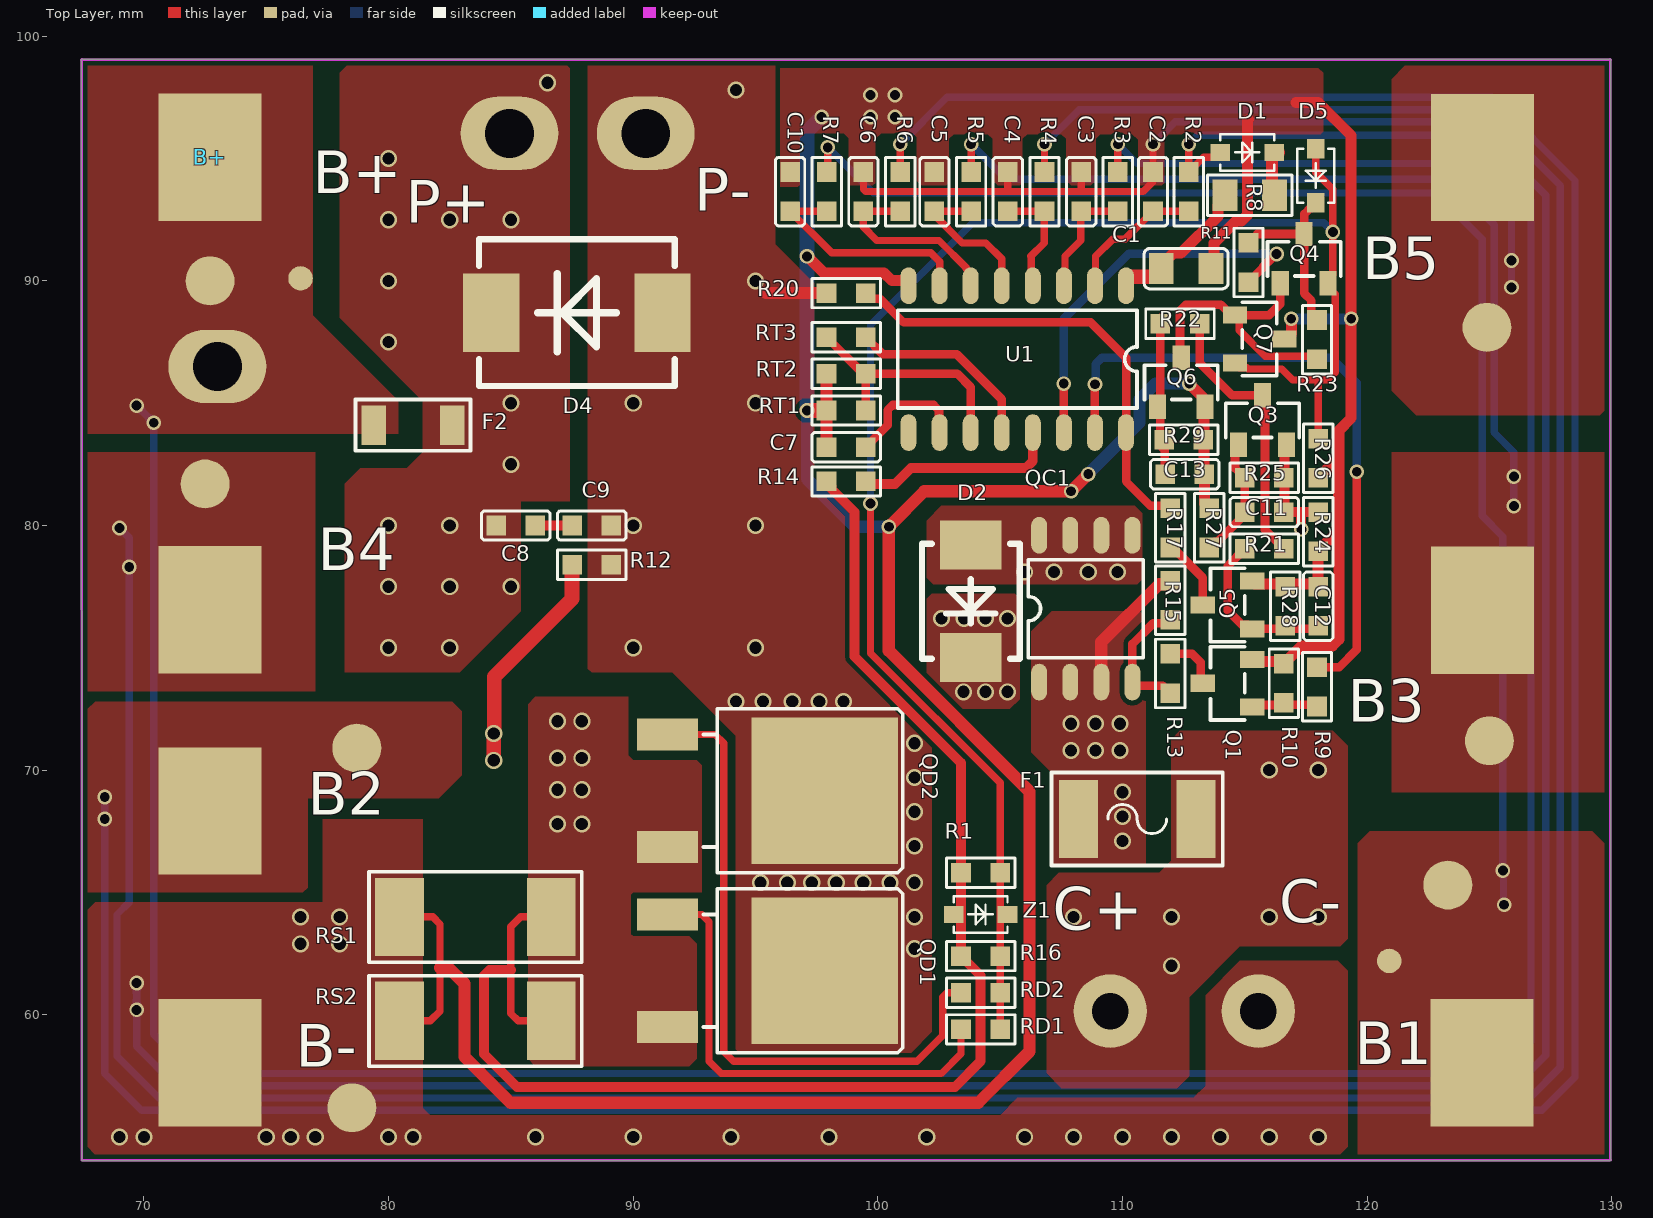
[diagram p0: Top Layer view]
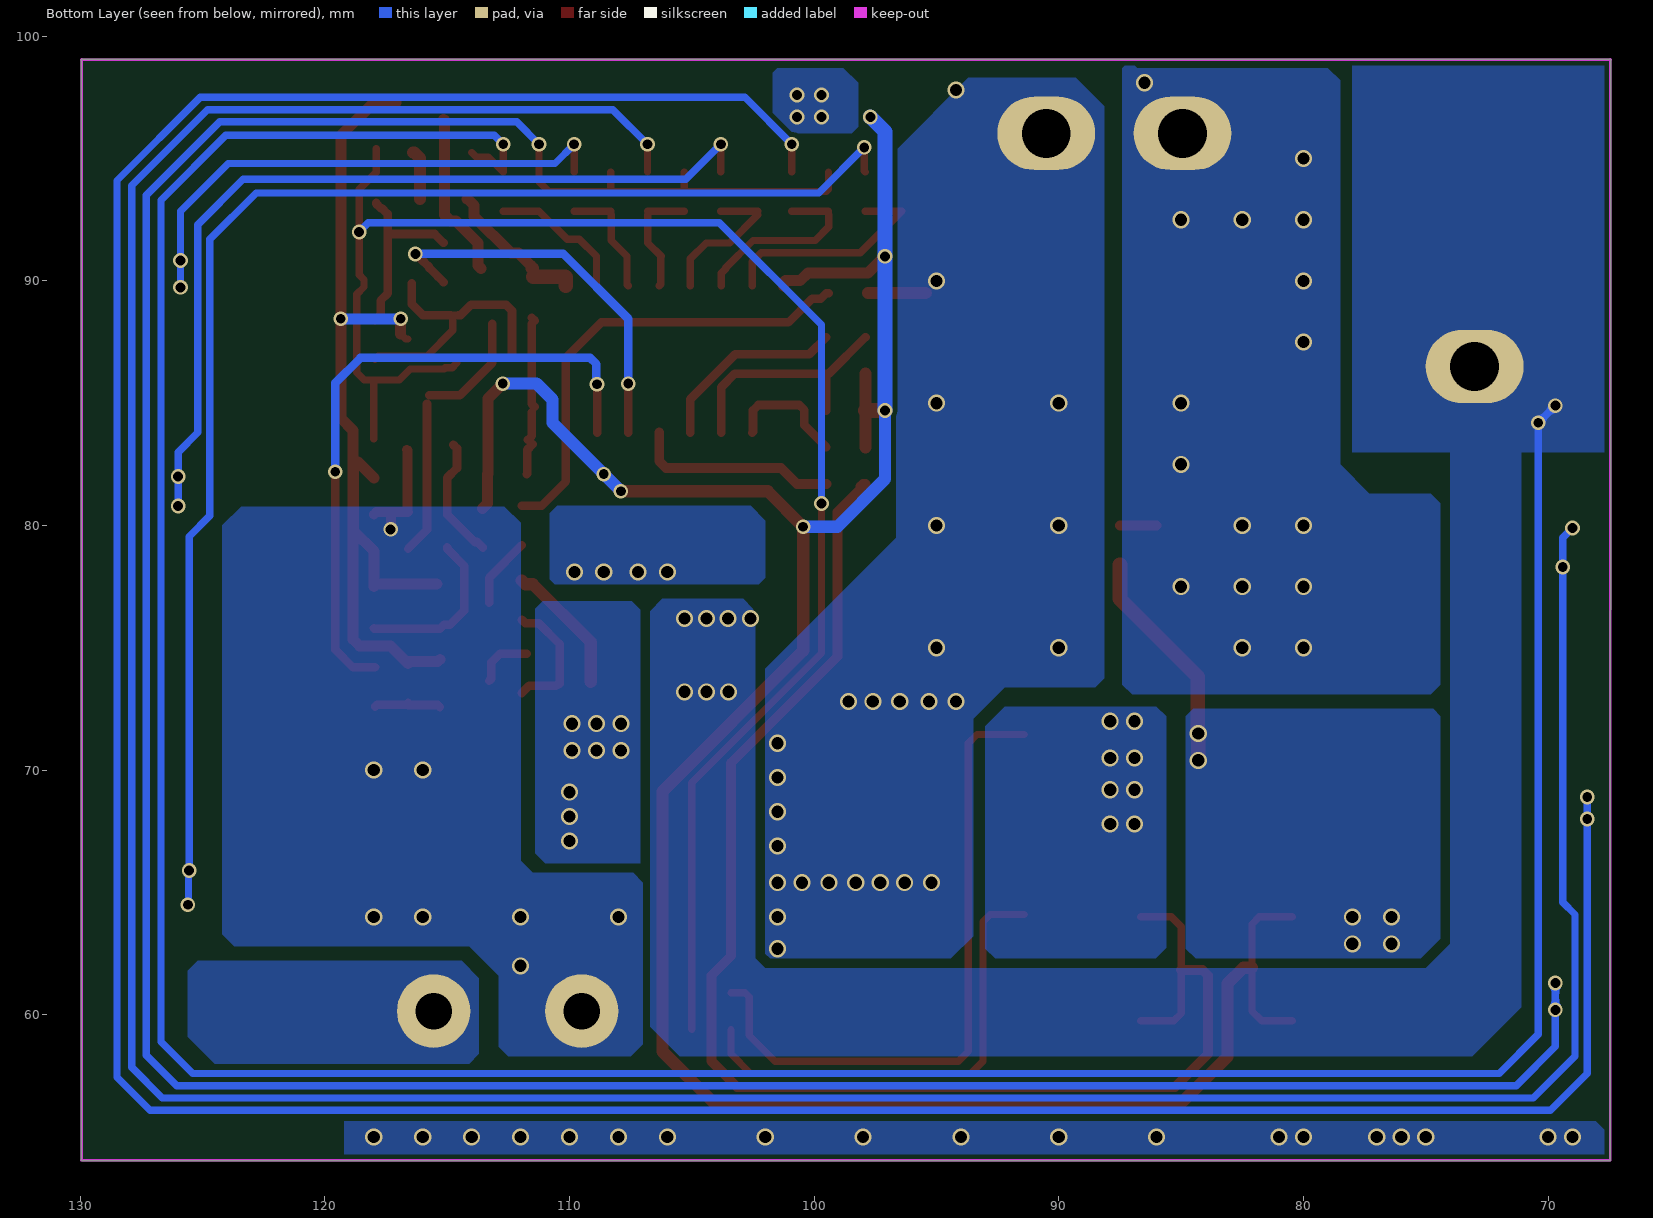
[diagram p1: Bottom Layer view, seen from below]
# Altium PCB MISC75736.PcbDoc
Units mm, origin at the board's own origin, x right, y up, seen from the top; angles counter-clockwise.
Board outline 62.51 x 45.01 mm, 2 copper layers (Top Layer, Bottom Layer); 76 components, 42 nets, 177 pads, 143 vias.

## Layer stack, top to bottom (the 12.6 mil dielectric is the usual default, probably not edited)
Top Solder: solder mask 0.0102, Solder Resist, Dk 3.5
Top Layer: signal copper 0.0356
Dielectric 1: dielectric 0.32, FR-4, Dk 4.8
Bottom Layer: signal copper 0.0356
Bottom Solder: solder mask 0.0102, Solder Resist, Dk 3.5

## Board outline
67.448,54.041 129.948,54.041 129.954,54.048 129.954,99.048 129.948,99.054 67.448,99.054 67.441,99.048

## Design rules (kind name [scope] priority, off if disabled: settings)
Clearance [All] p1: gap=0.2 ignorepadtopadclearanceinfootprint=FALSE
ComponentClearance [All] p1: gap=0 collisioncheckmode=3 verticalgap=0 showdistances=FALSE
HoleToHoleClearance [All] p1: gap=0 allowstackedmicrovias=TRUE
MinimumSolderMaskSliver [All] p1: minsoldermaskwidth=0
PlaneConnect [All] p1: planeconnectstyle=Direct reliefexpansion=0.508 reliefentries=4 reliefconductorwidth=0.254 reliefairgap=0.254
PolygonConnect [All] p1: connectstyle=Direct reliefconductorwidth=0.254 reliefentries=4 polygonreliefangle="90 Angle" airgapwidth=0.254
RoutingVias [All] p1: holewidth=0.4 width=0.6 viastyle="Through Hole" minholewidth=0.4 minwidth=0.6 maxholewidth=0.5 maxwidth=0.7
SilkToSilkClearance [All] p1: silktosilkclearance=0
SilkToSolderMaskClearance [IsPad] p1: minsilkscreentomaskgap=0 clearancetoexposedcopper=TRUE
SolderMaskExpansion [All] p1: expansion=0.102 istentingtop=FALSE
SupplyNets "Schematic Supply Nets_1" [InNet('P-')] p1: voltage=0.000
SupplyNets "Schematic Supply Nets" [InNet('B0')] p2: voltage=0.000
Width [All] p1: maxlimit=10 minlimit=0.254 preferedwidth=0.254
24 further rules are at their usual default settings.

## Components (designator, comment, footprint, x,y, rotation, side; value= is the part's Value field where it differs from the comment)
B1 "Pad" Pad10X8mm 124.7,58.039 r0 top
B2 "Pad" Pad10X8mm 72.698,68.326 r0 top
B3 "Pad" Pad10X8mm 124.714,76.535 r0 top
B4 "Pad" Pad10X8mm 72.698,76.552 r0 top
B5 "Pad" Pad10X8mm 124.714,95.043 r0 top
B+ "Pad" Pad10X8mm 72.698,95.052 r0 top
B+ "Pth" 4*3#1 73,86.5 r0 top
B- "Pad" Pad10X8mm 72.698,58.039 r0 top
C1 "1uF50V/805" C0805L 112.6,90.5 r180 top
C2 "0.1uF" C0603A 111.246,93.65 r270 top
C3 "0.1uF" C0603A 108.311,93.65 r270 top
C4 "0.1uF" C0603A 105.311,93.65 r270 top
C5 "0.1uF" C0603A 102.311,93.65 r270 top
C6 "0.1uF" C0603A 99.411,93.65 r270 top
C7 "0.1uF" C0603A 98.7,83.2 r180 top
C8 "0.1uF" C0603A 85.2,80 r0 top
C9 "0.1uF" C0603A 88.3,80 r0 top
C10 "0.1uF" C0603A 96.411,93.65 r270 top
C11 "0.1uF" C0603A 115.8,80.55 r180 top
C12 "NC" C0603A 118,76.7 r90 top
C13 "NC" C0603A 112.55,82.1 r0 top
C+ "Pth" 4*3#2 111.654,60.149 r0 top
C- "Pth" 4*3#3 115.552,60.149 r0 top locked
D1 "BAT46W" SOD323 115.1,95.25 r180 top
D2 "SS34" SMB(DO-214AA) 103.8,76.9 r90 top
D4 "RS5M" "SMC A(DO-214AB)" 87.7,88.7 r0 top
D5 "1N4148SW" SOD323 117.9,94.3 r90 top
F1 "PTC" F1812A 110.6,68 r0 top
F2 "F12F10 32V15A" R1206A 81,84.1 r0 top
P+ "Pth" 4*3#1 84.943,96.03 r0 top locked
P- "Pth" 4*3#1 90.511,96.03 r0 top locked
Q1 "MMBT5551" SOT23-3 114.3,73.55 r90 top
Q3 "MMBT5401" SOT23-3 115.725,84.3 r0 top
Q4 "MMBT5551" SOT23-3 117.425,90.9 r0 top
Q5 "MMBT5551" SOT23-3 114.3,76.75 r90 top
Q6 "MMBT5551" SOT23-3 112.4,85.85 r0 top
Q7 "MMBT5401" SOT23-3 115.6,87.625 r270 top
QC1 "P MOS*" SOP-8L(T3p) 108.5,76.6 r90 top
QD1 "N MOS*" TO-252 94.612,61.8 r270 top
QD2 "N MOS*" TO-252 94.612,69.158 r270 top
R1 "10M" R0603A 104.2,65.8 r0 top
R2 "1K" R0603A 112.711,93.65 r270 top
R3 "1K" R0603A 109.811,93.65 r270 top
R4 "1K" R0603A 106.811,93.65 r270 top
R5 "1K" R0603A 103.811,93.65 r270 top
R6 "1K" R0603A 100.911,93.65 r270 top
R7 "1K" R0603A 97.911,93.65 r270 top
R8 "1K/0805" R0805L 115.2,93.5 r180 top
R9 "100K" R0603A 117.95,73.4 r270 top
R10 "3.3M" R0603A 116.6,73.55 r270 top
R11 "1K" R0603A 115.15,90.75 r270 top
R12 "10M/NC" R0603A 88.3,78.4 r0 top
R13 "3.3M" R0603A 111.95,73.95 r270 top
R14 "1K" R0603A 98.7,81.8 r0 top
R15 "3M" R0603A 111.95,76.95 r90 top
R16 "10M/NC" R0603A 104.2,62.4 r0 top
R17 "0R" R0603A 111.95,79.9 r270 top
R20 "1K" R0603A 98.7,89.5 r0 top
R21 "1M" R0603A 115.8,79.05 r0 top
R22 "1M" R0603A 112.35,88.25 r0 top
R23 "1M" R0603A 117.95,87.6 r90 top
R24 "10K" R0603A 118,79.75 r90 top
R25 "10K" R0603A 115.8,81.95 r0 top
R26 "10M" R0603A 118,82.75 r90 top
R27 "100K" R0603A 113.55,79.9 r270 top
R28 "100K" R0603A 116.65,76.7 r270 top
R29 "100K" R0603A 112.5,83.5 r180 top
RD1 "47R" R0603A 104.2,59.4 r180 top
RD2 "47R" R0603A 104.2,60.9 r0 top
RS1 "R010" R2512L 83.55,64 r0 top
RS2 "R010" R2512L 83.55,59.75 r0 top
RT1 "10K B=3435" R0603A 98.7,84.7 r0 top
RT2 "10K B=3435" R0603A 98.7,86.2 r0 top
RT3 "1K" R0603A 98.7,87.7 r0 top
U1 "CM10D1*" SOP16L 105.7,86.8 r270 top
Z1 "15V" SOD323 104.2,64.1 r180 top

## Footprints (in the part's own frame and the unit in brackets; to place one, negate y for a bottom-side part, rotate by r counter-clockwise, add the part's x,y. Pads: shape width x height; smd on the part's side, far side on the other; paste and mask are expansions set on the pad)
4*3#1 [mm] "通孔焊盘"
  oval 4x3 hole 2 mask+0: 1(0,0)
4*3#2 [mm] "通孔焊盘"
  round 3 hole 1.5 mask+0: 1(-2.154,0)
4*3#3 [mm] "通孔焊盘"
  round 3 hole 1.5 mask+0: 1(0,0)
C0603A [mm] "贴片电容"
  rect 0.8x0.8 smd mask+0.08: 1(-0.8,0) 2(0.8,0)
  silkscreen extent -1.4,-0.6 1.4,0.6
C0805L [mil] "贴片电容"
  rect 40x50 smd paste+0 mask+1.97: 1(-40,0) 2(40,0)
  silkscreen extent -68,-32 68,32
F1812A [mm] "贴片电阻"
  rect 1.6x3.2 smd: 1(-2.4,0) 2(2.4,0)
  silkscreen extent -3.5,-1.9 3.5,1.9
Pad10X8mm [mm]
  rect 4.2x5.2 smd: 1(0,0)
R0603A [mm] "贴片电阻"
  rect 0.8x0.8 smd mask+0.08: 1(-0.8,0) 2(0.8,0)
  silkscreen extent -1.4,-0.6 1.4,0.6
R0805L [mil] "贴片电阻"
  rect 40x50 smd paste+0 mask+1.97: 1(-40,0) 2(40,0)
  silkscreen extent -68,-32 68,32
R1206A [mm] "贴片电阻"
  rect 1x1.6 smd: 1(-1.6,0) 2(1.6,0)
  silkscreen extent -2.35,-1.05 2.35,1.05
R2512L [mm] "贴片电阻"
  rect 2x3.2 smd: 1(-3.1,0) 2(3.1,0)
  silkscreen extent -4.35,-1.85 4.35,1.85
SMB(DO-214AA) [mm] "贴片二极管"
  rect 2x2.5 smd: 1(-2.3,0) 2(2.3,0)
  silkscreen extent -2.35,-2 2.35,2
"SMC A(DO-214AB)" [mm] "贴片二极管"
  rect 2.3x3.2 smd: 1(-3.5,0) 2(3.5,0)
  silkscreen extent -4,-3 4,3
SOD323 [mm] "贴片二极管"
  rect 0.8x0.7 smd: 1(-1.1,0) 2(1.1,0)
  silkscreen extent -1.1,-0.75 1.1,0.75
SOP16L [mm]
  oval 1.5x0.65 smd: 1(-3,4.445) 2(-3,3.175) 3(-3,1.905) 4(-3,0.635) 5(-3,-0.635) 6(-3,-1.905) 7(-3,-3.175) 8(-3,-4.445) 9(3,-4.445) 10(3,-3.175) 11(3,-1.905) 12(3,-0.635) 13(3,0.635) 14(3,1.905) 15(3,3.175) 16(3,4.445)
  silkscreen extent -2,-4.89 2,4.89
SOP-8L(T3p) [mm] "贴片MOS（非常规）"
  oval 1.5x0.65 smd: 1(-3,-1.905) 2(-3,-0.635) 2(-3,0.635) 2(-3,1.905) 3(3,-1.905) 3(3,-0.635) 3(3,0.635) 3(3,1.905)
  silkscreen extent -2,-2.35 2,2.35
SOT23-3 [mm] "贴片IC/MOS*"
  rect 0.7x1 smd: 1(-0.975,-1) 2(0.975,-1) 3(0,1.016)
  silkscreen extent -1.5,-0.7 1.5,0.7
TO-252 [mm]
  rect 1.3x2.5 smd: 1(-2.3,-3.212) 2(2.3,-3.212)
  rect 6x6 smd: 3(0,3.213)
  silkscreen extent -3.35,-1.75 3.35,6.4

## Part data
B1 B2 B3 B4 B5 B+ B-: "connection pad (non-through-hole)"
B+ C+ C- P+ P-: "through-hole pad"
C1 C2 C3 C4 C5 C6 C7 C8 C9 C10 C11 C12 C13: library part CAP, "chip capacitor"
D1 D4 D5: "chip diode"
D2: "chip Schottky diode"
F1: "chip resettable fuse"
F2: library part FUSE
Q1 Q3 Q4 Q5 Q6 Q7: "chip transistor"
QC1 QD1 QD2: "chip MOSFET"
R1 R2 R3 R4 R5 R6 R7 R8 R9 R10 R11 R12 R13 R14 R15 R16 R17 R20 R21 R22 R23 R24 R25 R26 R27 R28 R29 RD1 RD2 RT1 RT3: library part RES, "chip resistor"
RS1 RS2: library part RES2, "chip metal alloy resistor"
RT2: library part NTC, "chip thermistor"
U1: library part CM1061*, "6-cell battery protection IC"
Z1: "chip Zener diode"

## Free pads (board coordinates)
  round 2 smd: 1(72.5,81.7) 1(72.7,90) 1(78.5,56.2) 1(78.7,70.9) 1(123.3,65.3) 1(124.9,88.1) 1(125,71.2)
  round 1 smd: 1(76.4,90.1) 1(120.9,62.2)

## Via types
v1: diameter 0.7, hole 0.5, Top Layer to Bottom Layer, tented both sides, 102 vias
v2: diameter 0.6, hole 0.4, Top Layer to Bottom Layer, tented both sides, 41 vias

## Nets (pads, with @x,y where several pads share a name; then routed paths per layer and width w, separated by ;. In a path a pad name is that pad's centre, name@x,y a point inside that pad or via, vN(x,y) a via of type N, cw(c..) or ccw(c..) an arc to the next point about the centre after c; other vN are vias at no path point)
B0: B-.1 C1.1 C2.1 C3.1 C4.1 C5.1 C6.1 C7.2 C10.1 C12.2 C13.2 C-.1 pad.1@78.5,56.2 Q1.2 Q5.2 Q6.2 Q7.3 R10.1 R12.1 R24.1 R26.1 R27.1 R28.1 R29.1 RS1.1 RS2.1 RT1.1 RT2.1 U1.8 | length 295.3
  Top Layer w0.3: RS2.1 81.7,59.75 82.1,60.15 82.1,61.925 82.1,63.7 81.8,64 RS1.1 ; C6.1 99.411,93.75 99.511,93.65 105.311,93.65 ; C4.1 105.311,93.65 ; C3.1 108.311,93.65 ; v2(111.246,95.585) C2.1 111.246,94.05 110.846,93.65 108.311,93.65 ; Q7.3 116.7,87.625 Q7.3@116.9,87.825 ; 105.311,93.65 108.311,93.65
  Top Layer w0.45: v2(97.1,91) 97.129,91 97.804,90.325 100.256,90.325 100.569,90.013 101.163,90.013 101.255,89.92 U1.8 ; v2(112.725,85.8) 113.325,85.2 113.325,85.05 113.338,85.037 113.338,82.113 C13.2 113.35,80.9 R27.1 ; C1.1 113.745,90.629 113.745,91.546 114.639,92.44 114.868,92.44 115.117,92.689 115.117,96.567 115.15,96.6 ; Q1.2 115.387,74.437 116.513,74.437 R10.1 117.325,75.075 118.576,75.075 118.85,75.349 118.85,83.888 119.35,84.388 v2(119.35,88.45) 119.35,95.95 118,97.3 117.1,97.3 ; Q5.2@115.425,77.6 115.438,77.612 117.888,77.612 C12.2 R24.1@118,78.85 ; Q7.3@116.9,87.825 v2(116.9,88.45) ; R24.1 118.825,79.775 118.825,82.4 ; R26.1 118.65,82.6
  Top Layer w0.5: 82.1,61.925 82.45,61.925 83.1,61.275 83.1,58.281 84.981,56.4 104.1,56.4 106.2,58.5 106.2,69.126 100.45,74.876 v2(100.45,79.95) 101.9,81.4 v2(107.9,81.4) v2(108.6,82.1) ; C7.2 RT1.1 RT2.1
  Top Layer w0.6: v1(84.3,70.4) v1(84.3,71.5) 84.319,71.519 84.319,73.819 87.5,77 R12.1 ; v2(97.1,84.7) RT1.1
  Bottom Layer w0.3: v2(69.7,60.2) 69.7,58.704 71.304,57.1 126.05,57.1 127.299,58.349 127.299,93.501 124.3,96.5 112.161,96.5 v2(111.246,95.585) ; v2(69.7,60.2) v2(69.7,61.3)
  Bottom Layer w0.45: v2(116.9,88.45) v2(119.35,88.45)
  Bottom Layer w0.5: v2(97.1,84.7) 97.1,81.9 99.05,79.95 v2(100.45,79.95) ; v2@107.987,81.487 110.7,84.2 110.7,85.15 111.35,85.8 v2(112.725,85.8)
  Bottom Layer w0.6: v2(97.1,84.7) 97.1,96.1 v2(97.7,96.7)
  other v1: 69,55 70,55 75,55 76,55 77,55 80,55 81,55 86,55 90,55 94,55 98,55 102,55 106,55 108,55 110,55 112,55 114,55 116,55 118,55 76.4,62.9 78,62.9 76.4,64 78,64
  other v2: 99.7,96.7 100.7,96.7 99.7,97.6 100.7,97.6
B1: B1.1 pad.1@120.9,62.2 pad.1@123.3,65.3 R7.1 | length 56.9
  Top Layer w0.3: R7.1 97.956,94.494 v2(97.956,95.456)
  Bottom Layer w0.3: v2(97.956,95.456) 99.817,93.595 122.805,93.595 124.7,91.7 124.7,80.4 125.55,79.55 v2(125.55,65.9) 125.575,65.875 125.575,64.525 v2(125.6,64.5)
B2: B2.1 pad.1@78.7,70.9 R6.1 | length 140.2
  Top Layer w0.3: R6.1 v2(100.911,95.585)
  Bottom Layer w0.3: v2(68.4,68.9) v2(68.4,68) 68.4,57.6 69.9,56.1 127.15,56.1 128.5,57.45 128.5,94.1 125.1,97.5 102.826,97.5 v2(100.911,95.585)
B3: B3.1 pad.1@125,71.2 R5.1 | length 35.7
  Top Layer w0.3: R5.1 v2(103.811,95.585)
  Bottom Layer w0.3: v2(103.811,95.585) 105.246,94.15 123.35,94.15 125.2,92.3 125.2,83.8 126,83 v2(126,82) v2(126,80.8)
B4: B4.1 pad.1@72.5,81.7 R4.1 | length 142.3
  Top Layer w0.3: R4.1 v2(106.811,95.585)
  Bottom Layer w0.3: v2(69,79.9) 69.4,79.5 v2(69.4,78.3) 69.4,64.6 68.9,64.1 68.9,58.3 70.6,56.6 126.65,56.6 127.9,57.85 127.9,93.9 124.8,97 108.226,97 v2(106.811,95.585)
B5: B5.1 pad.1@124.9,88.1 R3.1 | length 21.5
  Top Layer w0.3: R3.1 v2(109.811,95.585)
  Bottom Layer w0.3: v2(109.811,95.585) 110.596,94.8 123.95,94.8 125.9,92.85 v2(125.9,90.833) v2(125.9,89.733)
B+: B+.1 D1.2 D2.1 F2.1 pad.1@72.7,90 pad.1@76.4,90.1 R2.1 | length 135.9
  Top Layer w0.3: v2(112.711,95.585) R2.1 113.311,95.05 113.8,95.05 D1.2
  Bottom Layer w0.3: v2(69.7,84.9) v2(70.4,84.2) 70.4,59.2 72,57.6 125.4,57.6 126.7,58.9 126.7,93.3 124.05,95.95 113.076,95.95 v2(112.711,95.585)
  other v1: 103.5,73.2 104.4,73.2 105.3,73.2 102.6,76.2 103.525,76.2 104.4,76.2 105.3,76.2
C+: C11.1 C+.1 F1.2 Q3.2 R24.2 R25.2 | length 4.7
  Top Layer w0.4: C11.1 C11.1@116.625,80.55 ; Q3.2@116.65,83.1 116.625,83.075 116.625,81.9 C11.1@116.625,80.55 ; v2(117.313,79.84) 117.3,79.853 117.3,80.55 ; R24.2@118,80.45 117.9,80.55 117.3,80.55 ; C11.1@116.625,80.55 117.3,80.55
  other v1: 112,62 108,64 112,64 116,64 118,64 116,70 118,70
D0: D5.1 Q4.3 R11.1 R23.2 | length 7.7
  Top Layer w0.35: R11.1 115.516,91.916 Q4.3 ; D5.1 117.9,93.15 117.725,92.975 117.675,92.975 117.436,92.736 117.436,91.927 Q4.3 ; R23.2 117.725,88.625 117.725,89.195 117.425,89.495 Q4.3
D01: D5.2 Q4.2 Q7.2 R1.2 R16.2 R26.2 RD1.1 RD2.2 Z1.1 | length 68.3
  Top Layer w0.3: v2(99.7,80.9) 99.7,74.778 105,69.478 R1.2 105,64.1 R16.2 RD2.2 RD1.1 ; Q7.2 114.8,86.45 115.076,86.45 115.126,86.4 116.51,86.4 116.96,85.95 118.013,85.95 ; D5.2 117.9,94.445 118.6,93.745 v2(118.6,91.997) 118.6,90.25 118.4,90.05 Q4.2 118.4,89.75 118.7,89.45 118.7,86.255 118.395,85.95 118.013,85.95 ; R26.2 118,85.937 118.013,85.95
  Bottom Layer w0.3: v2(99.7,80.9) 99.7,88.2 103.875,92.375 118.222,92.375 v2(118.6,91.997)
NetC7_1: C7.1 U1.10 | length 5.1
  Top Layer w0.35: C7.1 100.4,84.1 100.4,84.72 100.605,84.925 102.275,84.925 102.499,84.701 102.499,83.826 U1.10
NetC8_1: C8.1 D4.1 F2.2 P+.1
  other v1: 80,75 82.5,75 80,77.5 82.5,77.5 85,77.5 80,80 82.5,80 85,82.5 85,85 80,87.5 80,90 80,92.5 82.5,92.5 85,92.5 80,95 86.5,98.1
NetC8_2: C8.2 C9.1 | length 1.5
  Top Layer w0.4: C8.2 C9.1
NetC11_2: C11.2 Q3.1 R25.1 R27.2 | length 5
  Top Layer w0.35: R27.2 113.775,79.325 113.875,79.325 C11.2@115,80.45 ; Q3.1 114.6,83.15 114.6,82.35 R25.1 C11.2
NetC12_1: C12.1 Q5.1 R21.1 R28.2 | length 6.9
  Top Layer w0.35: R21.1@114.975,79.075 R21.1@115,79.1 ; R21.1 114.3,78.35 114.3,76.525 114.875,75.95 115.125,75.95 Q5.1 115.312,75.787 117.988,75.787 C12.1@118,75.8
NetC13_1: C13.1 Q6.1 R22.1 R29.2 | length 6.1
  Top Layer w0.35: Q6.1 111.55,84.975 R22.1 ; R22.1@111.425,88.375 R22.1@111.55,88.5 ; R29.2@111.512,83.313 111.725,83.1 111.725,82.125 C13.1 ; Q6.1@111.537,84.638 111.537,83.662 R29.2
NetD1_1: D1.1 R8.1 | length 2
  Top Layer w0.5: R8.1@116.116,93.35 116.116,95.016 116.35,95.25 D1.1@116.4,95.25
NetD2_2: D2.2 QC1.3
  other v1: 106,78.1 107.2,78.1 108.6,78.1 109.8,78.1
NetF1_1: F1.1 QC1.2 R15.2 | length 5.5
  Top Layer w0.5: QC1.2@109.135,73.6 109.135,75.235 111.5,77.6 111.8,77.6 R15.2
  other v1: 110,67.1 110,68.1 110,69.1 107.9,70.8 108.9,70.8 109.9,70.8 107.9,71.9 108.9,71.9 109.9,71.9
NetQ1_1: Q1.1 R9.2 R10.2 | length 2.7
  Top Layer w0.35: Q1.1 115.388,72.662 R10.2@116.6,72.662 ; R10.2 116.675,72.675 117.875,72.675 R9.2
NetQ1_3: Q1.3 R13.1 | length 2.4
  Top Layer w0.35: R13.1@111.75,74.75 R13.1 112.85,74.75 113.2,74.4 113.2,73.734 Q1.3@113.284,73.65
NetQ3_3: Q3.3 R21.2 R22.2 | length 11
  Top Layer w0.35: R22.2 113.15,86.65 114.484,85.316 Q3.3 ; Q3.3@115.825,84.966 115.825,79.825 R21.2
NetQ4_1: Q4.1 Q6.3 Q7.1 R23.1 | length 11.4
  Top Layer w0.3: Q7.1@114.55,88.6 Q7.1@114.7,88.6 ; Q7.1@114.85,88.6 Q7.1@114.7,88.6 ; R23.1 117.825,86.925 115.825,86.925 114.774,87.976 114.774,88.526 Q7.1@114.7,88.6
  Top Layer w0.35: Q6.3@112.35,87.066 112.35,88.78 112.595,89.025 114.025,89.025 114.45,88.6 Q7.1@114.55,88.6 ; Q7.1@114.85,88.6 116,88.6 116.45,89.05 Q4.1
NetQ5_3: Q5.3 R17.2 | length 2.9
  Top Layer w0.35: R17.2@111.95,79.2 113.284,77.866 Q5.3@113.284,76.85
NetQC1_1: QC1.1 R13.2 R15.1 | length 5.3
  Top Layer w0.35: QC1.1@110.405,73.539 110.405,75.155 111.254,76.004 111.804,76.004 R15.1 ; QC1.1 110.405,73.589 110.544,73.45 111.65,73.45 R13.2
NetQD1_1: QD1.1 RD1.2 | length 19.4
  Top Layer w0.3: QD1.1 92.8,64.1 93.1,63.8 93.1,58.1 93.6,57.6 102.6,57.6 103.4,58.4 RD1.2
NetQD1_2: QD1.2 QD2.2 R1.1 R14.1 R16.1 RS1.2 RS2.2 Z1.2 | length 59.1
  Top Layer w0.3: RS2.2 85.3,59.75 85,60.05 85,61.825 85,63.6 85.4,64 RS1.2
  Top Layer w0.4: 85,61.825 84.125,61.825 83.9,61.6 83.9,58.4 85.25,57.05 103.15,57.05 104.2,58.1 104.2,61.6 R16.1 103.4,64.1 R1.1 103.4,70.3 99.05,74.65 99.05,80.55 98.1,81.5 98.1,81.6 98,81.7 R14.1@97.9,81.7
  other v1: 86.9,67.8 87.9,67.8 86.9,69.2 87.9,69.2 86.9,70.5 87.9,70.5 86.9,72 87.9,72
NetQD2_1: QD2.1 RD2.1 | length 27
  Top Layer w0.3: QD2.1 93.342,71.458 93.7,71.1 93.7,58.5 94.1,58.1 101.6,58.1 102.65,59.15 102.65,60.724 102.826,60.9 RD2.1
NetR9_1: R9.1 U1.15 | length 26.8
  Top Layer w0.35: U1.15 v2(108.875,85.775) ; R9.1 118.85,74.2 119.575,74.925 v2(119.575,82.2)
  Bottom Layer w0.35: v2(108.875,85.775) 108.9,85.8 108.9,86.6 109.15,86.85 118.55,86.85 119.575,85.825 v2(119.575,82.2)
NetR11_2: R11.2 U1.14 | length 16.1
  Top Layer w0.35: v2(107.6,85.8) 107.603,85.798 107.603,83.802 U1.14 ; R11.2 115.375,90.175 115.725,90.525 115.725,90.555 115.945,90.775 115.97,90.775 116.295,91.1 v2(116.3,91.1)
  Bottom Layer w0.35: v2(107.6,85.8) 107.6,88.45 110.25,91.1 v2(116.3,91.1)
NetR14_2: R14.2 U1.13 | length 8.4
  Top Layer w0.4: R14.2@99.5,81.7 100.7,81.7 101.35,82.35 106.05,82.35 106.335,82.635 U1.13
NetRT1_2: RT1.2 RT2.2 RT3.1 U1.11 | length 10.1
  Top Layer w0.35: RT3.1 99.4,86.2 RT2.2 ; RT1.2 RT2.2 ; U1.11 103.795,85.655 103.25,86.2 RT2.2
NetRT3_2: RT3.2 U1.12 | length 8
  Top Layer w0.35: RT3.2 100.2,87 103.228,87 105.065,85.163 U1.12
P-: C9.2 D4.2 P-.1 QD1.3 QD2.3 R12.2 R20.1 | length 2.4
  Top Layer w0.5: 95.441,89.5 R20.1@97.8,89.5
  other v1: 101.5,62.7 101.5,64 95.2,65.4 96.3,65.4 97.3,65.4 98.3,65.4 99.4,65.4 100.5,65.4 101.5,65.4 101.5,66.9 101.5,68.3 101.5,69.7 101.5,71.1 94.2,72.8 95.3,72.8 96.5,72.8 97.6,72.8 98.6,72.8 90,75 95,75 90,80 95,80 90,85 95,85 95,90 94.2,97.8
VC1: C2.2 R2.2 U1.2 | length 5.8
  Top Layer w0.3: U1.2 108.9,89.825 108.9,91 109.6,91.7 110.096,91.7 C2.2 R2.2
VC2: C3.2 R3.2 U1.3 | length 4.7
  Top Layer w0.3: U1.3 107.65,89.845 107.65,91 108.3,91.65 C3.2@108.3,92.7 ; C3.2 R3.2
VC3: C4.2 R4.2 U1.4 | length 4.7
  Top Layer w0.3: C4.2 R4.2 ; U1.4 106.268,89.867 106.268,90.982 106.25,91 106.8,91.55 R4.2@106.8,92.7
VC4: C5.2 R5.2 U1.5 | length 6.1
  Top Layer w0.3: C5.2@102.3,92.7 103.45,91.55 104.415,91.55 105.065,90.9 U1.5 ; C5.2 R5.2
VC5: C6.2 R6.2 U1.6 | length 7.7
  Top Layer w0.3: C6.2@99.4,92.7 99.4,92.21 99.96,91.65 102.5,91.65 103.62,90.53 103.62,90.495 103.8,90.315 U1.6@103.8,89.805 ; C6.2 R6.2
VC6: C10.2 R7.2 U1.7 | length 9.5
  Top Layer w0.3: R7.2 C10.2 98.111,91.15 102.163,91.15 102.525,90.788 U1.7
VCC: C1.2 R8.2 U1.1 | length 6.1
  Top Layer w0.45: C1.2@111.476,90.165 C1.2@111.476,90.519 ; C1.2 111.584,90.627 112.092,91.135 112.397,91.135 113.901,92.639 113.901,93.09 114.161,93.35 R8.2@114.184,93.35
  Top Layer w0.6: U1.1@110.155,89.81 110.155,90.151 110.168,90.165 C1.2@111.476,90.165
VM: R17.1 R20.2 U1.16 | length 19.1
  Top Layer w0.35: R20.2@99.4,89.5 R20.2 99.725,89.275 100.075,89.275 101.05,88.3 108.7,88.3 110.145,86.855 U1.16 110.145,81.8 111.145,80.8 R17.1@111.95,80.8
pads on no net: U1.9

## Polygon pours and split planes (outlines as drawn)
C+ on Top Layer "Top Layer-C+" (solid, pour order 58): 112,71.25 112.35,71.6 118.6,71.6 119.2,71 119.2,67.65 119.2,63.1 118.9,62.8 114.8,62.8 112.72,60.72 112.72,57.485 112.235,57 107.5,57 106.9,57.6 106.9,65.3 107.4,65.8 111.5,65.8 112,66.3
B5 on Top Layer "Top Layer-B5" (solid, pour order 10): 121,85.5 122,84.5 123.9,84.5 124.85,84.5 129.5,84.5 129.948,84.948 129.948,99.035 124.781,99.035 121.785,99.035 121,98.25
NetC8_1 on Top Layer "Top Layer-NetC8_1" (solid, pour order 22): 83.9,99 83.852,99.048 78.548,99.048 78,98.5 78,88.489 81.4,85.089 81.4,83 80.733,82.333 78.833,82.333 78.2,81.7 78.2,74 78.3,74 79.1,74 82.9,74 85.4,76.5 85.4,81 87.4,81 87.4,98.7 87.1,99
B0 on Top Layer "Top Layer-B0" (solid, pour order 0): 113.4,60.8 113.4,57.1 112.9,56.6 105.7,56.6 105,55.9 81.7,55.9 81.4,56.2 81.4,61.35 81.4,68 77.3,68 77.3,64.6 68,64.6 67.6,64.2 67.6,54.7 68,54.3 118.9,54.3 119.2,54.6 119.2,61.8 118.8,62.2 114.8,62.2
B2 on Top Layer "Top Layer-B2" (solid, pour order 2): 76.7,65.2 76.5,65 67.448,65 67.448,66.9 67.448,72.248 68,72.8 82.6,72.8 83,72.4 83,69.8 82.05,68.85 76.7,68.85
NetQD1_2 on Top Layer "Top Layer-NetQD1_2" (solid, pour order 14): 90,63.2 89.9,63.3 89.9,64.9 90,65 92.8,65 92.8,70.2 92.6,70.4 90,70.4 89.8,70.6 89.8,71.8 89.8,73 86,73 85.7,72.7 85.7,58.2 86,57.9 92.3,57.9 92.6,58.2 92.6,62.9 92.3,63.2
B+ on Top Layer "B+_L01_P066" (solid, pour order 66): 80.4,83.75 80.4,85.1 79.8,85.7 76.9,88.6 76.9,98.9 77,99 76.955,99.045 67.448,99.045 67.448,83.75
P- on Top Layer "Top Layer-P-" (solid, remove dead copper, pour order 18): 97.4,83.65 97.4,81.95 99.65,79.7 99.65,73.67 100.62,72.7 102.2,71.121 102.2,59.3 101.3,58.4 94.4,58.4 94.2,58.6 94.2,71.4 91.6,74 88.3,74 88.148,74.152 88.148,99.048 95.545,99.048 95.8,98.793 95.8,91.5 97.4,89.9
B+ on Top Layer "Top Layer-B+ 2" (solid, pour order 52): 102,73.9 103.4,72.5 105.4,72.5 105.8,72.9 105.8,77 105.6,77.2 102.2,77.2 102,77
B0 on Top Layer "Top Layer-B0 2" (solid, remove dead copper, pour order 44): 118.113,96 118.2,96.087 118.2,98.5 118,98.7 117.3,98.7 97.4,98.7 95.35,98.7 95.2,98.55 95.2,94.05 95.4,93.85 96.733,93.85 96.8,93.917 96.8,95.8 97.03,96.03 98.6,96.03 98.8,95.83 98.8,93.9 99.8,93.9 99.9,94 99.9,95.8 100.13,96.03 101.435,96.03 101.6,95.865 101.6,94.1 101.8,93.9 102.8,93.9 102.9,94 102.9,95.8 103.1,96 104.5,96 104.7,95.8 104.7,94.1 104.9,93.9 105.8,93.9 105.9,94 105.9,95.8 106.1,96 107.5,96 107.7,95.8 107.7,94.1 107.9,93.9 108.7,93.9 108.9,94.1 108.9,95.8 109.1,96 110.4,96 110.635,95.765 110.635,94 110.735,93.9 111.6,93.9 111.7,94 111.7,95.8 111.9,96 114.6,96
NetF1_1 on Top Layer "Top Layer-NetD3_2" (solid, remove dead copper, pour order 30): 107.1,76.5 106.27,75.67 106.27,70.73 107.1,69.9 107.1,66.1 110.95,66.1 110.95,76.25 110.7,76.5
NetD2_2 on Top Layer "Top Layer-NetD2_2" (solid, pour order 28): 102,80.2 102.6,80.8 110.5,80.8 110.8,80.5 110.8,77.8 110.6,77.6 102.255,77.6 102,77.855
B3 on Top Layer "Top Layer-B3" (solid, pour order 8): 121,69.1 129.962,69.1 129.962,83 121,83
B1 on Top Layer "Top Layer-B1" (solid, pour order 6): 119.614,54.048 129.948,54.048 129.948,66.752 129.2,67.5 120.1,67.5 119.614,67.014
B4 on Top Layer "Top Layer-B4" (solid, pour order 4): 67.448,73.226 77,73.226 77,83 67.448,83 67.448,75.126
P- on Bottom Layer "Bottom Layer-P-" (solid, pour order 40): 102,74.143 96.641,79.502 96.641,95.359 93.7,98.3 89.3,98.3 88.148,97.148 88.148,73.752 88.516,73.384 92.216,73.384 93.5,72.1 93.5,63.213 94.413,62.3 101.8,62.3 102,62.5
B0 on Bottom Layer "NONET_L-01_P-001" (solid, remove dead copper, pour order 68): 125.195,62.205 125.6,61.8 125.6,59.1 124.5,58 114.1,58 113.7,58.4 113.7,61.5 114.405,62.205
B0 on Bottom Layer "NONET_L-01_P-001" (solid, remove dead copper, pour order 69): 68.053,55.65 67.703,55.3 67.7,55.3 67.7,54.1 67.8,54 118.9,54 119.2,54.3 119.2,55.65
C+ on Bottom Layer "Bottom Layer-C+" (solid, pour order 56): 112,80.105 112.669,80.774 123.426,80.774 124.2,80 124.2,63.3 123.7,62.8 114.1,62.8 112.9,61.6 112.9,58.7 112.5,58.3 107.5,58.3 107,58.8 107,61.45 107,65.4 107.4,65.8 111.5,65.8 112,66.3
NetD2_2 on Bottom Layer "Top Layer-NetD2_2" (solid, pour order 67): 102,80.2 102.6,80.8 110.5,80.8 110.8,80.5 110.8,77.8 110.6,77.6 102.255,77.6 102,77.855
B+ on Bottom Layer "Bottom Layer-B+" (solid, pour order 50): 71.1,60.3 73.1,58.3 105.5,58.3 106.7,59.5 106.7,76.5 106.2,77 102.9,77 102.5,76.6 102.4,76.3 102.4,62.3 102,61.9 75,61.9 74,62.9 74,83.3 73.8,83.5 71.3,83.5 71.1,83.3
B0 on Bottom Layer "Bottom Layer-B0" (solid, remove dead copper, pour order 64): 98.47,96.03 98.2,96.3 98.2,98.1 98.8,98.7 101.5,98.7 101.7,98.5 101.7,96.23 101.5,96.03
B0 on Bottom Layer "Bottom Layer-B0 1" (solid, pour order 38): 74.4,68.225 74.4,63.1 75.2,62.3 84.4,62.3 84.8,62.7 84.8,72.2 84.5,72.5 74.7,72.5 74.4,72.2
NetF1_1 on Bottom Layer "Top Layer-NetD3_2" (solid, remove dead copper, pour order 54): 111.4,66.6 111,66.2 107.1,66.2 107.1,76.55 107.45,76.9 111.1,76.9 111.4,76.6
NetQD1_2 on Bottom Layer "Bottom Layer-NetQD1_2" (solid, pour order 36): 85.6,69.145 85.6,62.738 86.037,62.3 92.6,62.3 93,62.7 93,71.8 92.2,72.6 86.007,72.6 85.6,72.193
NetC8_1 on Bottom Layer "Bottom Layer-NetC8_1" (solid, pour order 34): 79,98.7 78.5,98.2 78.5,82.5 77.3,81.3 74.8,81.3 74.4,80.9 74.4,73.5 74.8,73.1 87,73.1 87.4,73.5 87.4,98.7 87.1,99 86.8,98.7
B+ on Bottom Layer "Bottom Layer-B+ 1" (solid, remove dead copper, pour order 32): 67.448,89.2 67.448,99.048 77.952,99.048 78,99 78,83 67.548,83 67.448,83.1

## Keep-outs
Keep-Out Layer:
  circle w0.1: c67.448,99.048 r0.003
  circle w0.1: c129.948,54.048 r0.003
  circle w0.1: c129.948,99.048 r0.003
  circle w0.1: c129.948,99.048 r0.003
  lines w0.1: 67.448,54.048 129.948,54.048 129.948,99.048 67.448,99.048 67.448,54.048

## Silkscreen, mask and mechanical layers (free items; w line width, h text height)
Mechanical 1:
  circle w0.013: c84.943,96.03 r1.523
  circle w0.013: c90.511,96.03 r1.523
  circle w0.013: c115.552,60.149 r1.066
  circle w0.013: c111.654,60.149 r1.066
  lines w0.013: 70.596,58.039 74.803,58.039 ; 70.596,68.326 74.799,68.326 ; 70.596,76.552 74.799,76.552 ; 70.596,95.052 74.799,95.052 ; 72.698,92.451 72.698,97.654 ; 77.798,53.1 77.798,105.451 ; 119.614,55.441 119.614,97.628 ; 122.596,95.043 126.799,95.043 ; 122.6,58.039 126.799,58.039 ; 122.634,76.543 126.799,76.543 ; 70.596,55.451 74.799,55.451 74.799,60.654 70.596,60.654 70.596,55.451 ; 70.596,65.746 74.799,65.746 74.799,70.949 70.596,70.949 70.596,65.746 ; 70.596,73.951 74.799,73.951 74.799,79.154 70.596,79.154 70.596,73.951 ; 70.596,92.451 74.799,92.451 74.799,97.654 70.596,97.654 70.596,92.451 ; 122.596,55.441 126.799,55.441 126.799,60.645 122.596,60.645 122.596,55.441 ; 122.596,73.941 126.799,73.941 126.799,79.145 122.596,79.145 122.596,73.941 ; 122.596,92.441 126.799,92.441 126.799,97.645 122.596,97.645 122.596,92.441
  text "B5" at 121.525,93.982 h1.5 r90
  text "B+" at 77.39,93.737 h1.5 r90
  text "P+" at 84.396,92.122 h1.5
  text "P-" at 90.038,91.969 h1.5
  text "B3" at 125.313,79.704 h1.5 r90
  text "B4" at 78.09,75.198 h1.5 r90
  text "B2" at 77.89,67.184 h1.5 r90
  text "B-" at 72.2,59.3 h1.5
  text "B1" at 121.762,57.014 h1.5 r90
  text "C-" at 114.623,56.637 h1.5
  text "C+" at 109.982,56.485 h1.5